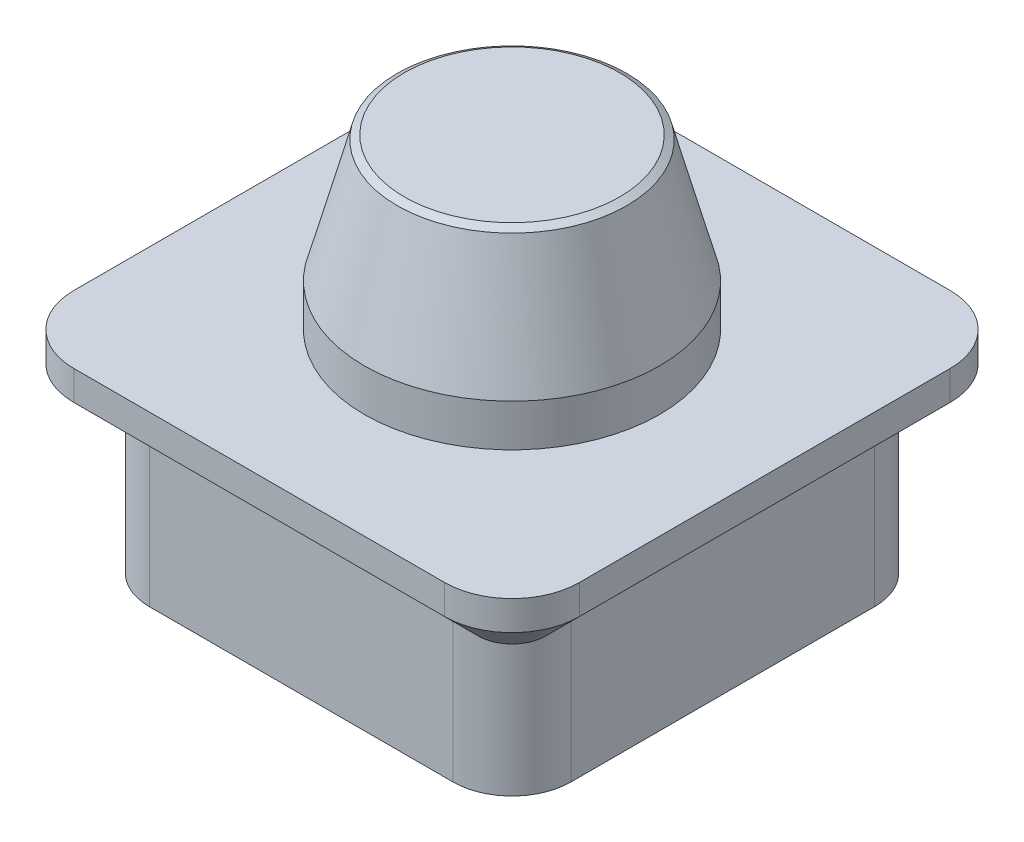
from build123d import *

# Parameters (mm, degrees)
CHAMFER_1_SIZE  = 1
CHAMFER_1_SIZE2 = 1.414213562
EXTRUDE_1_DEPTH = 15
EXTRUDE_2_DEPTH = 35
CHAMFER_2_SIZE  = 8


with BuildPart() as part:
    # 草图1 → 旋转1 (revolve)
    with BuildSketch(Plane.XY, mode=Mode.PRIVATE) as revolve_1_sk:
        Polygon((0, 0), (35, 0), (35, 10), (26.961524227, 40), (0, 40), align=None)
    revolve(revolve_1_sk.sketch.rotate(Axis((0, 40, 0), (0, -1, 0)), 180), axis=Axis((0, 40, 0), (0, -1, 0)))

    # 倒角1
    chamfer_1_edges = [part.edges().sort_by_distance(p)[0] for p in [
        (26.961524227, 40, 0),
    ]]
    chamfer_1_side = [part.faces().sort_by_distance(p)[0] for p in [
        (30.980762114, 25, 0),
    ]]
    chamfer(chamfer_1_edges, length=CHAMFER_1_SIZE, length2=CHAMFER_1_SIZE2, reference=chamfer_1_side[0])

    # 草图2 → 凸台-拉伸1 (add)
    with BuildSketch(Plane.XZ):
        with BuildLine():
            Line((44, -60), (-44, -60))
            ThreePointArc((-44, -60), (-55.313708499, -55.313708499), (-60, -44))
            Line((-60, -44), (-60, 44))
            ThreePointArc((-60, 44), (-55.313708499, 55.313708499), (-44, 60))
            Line((-44, 60), (44, 60))
            ThreePointArc((44, 60), (55.313708499, 55.313708499), (60, 44))
            Line((60, 44), (60, -44))
            ThreePointArc((60, -44), (55.313708499, -55.313708499), (44, -60))
        make_face()
    extrude(amount=EXTRUDE_1_DEPTH)

    # 草图3 → 凸台-拉伸2 (add)
    with BuildSketch(Plane.XZ.offset(15)):
        with BuildLine():
            Line((36, -50), (-36, -50))
            ThreePointArc((-36, -50), (-45.899494937, -45.899494937), (-50, -36))
            Line((-50, -36), (-50, 36))
            ThreePointArc((-50, 36), (-45.899494937, 45.899494937), (-36, 50))
            Line((-36, 50), (36, 50))
            ThreePointArc((36, 50), (45.899494937, 45.899494937), (50, 36))
            Line((50, 36), (50, -36))
            ThreePointArc((50, -36), (45.899494937, -45.899494937), (36, -50))
        make_face()
    extrude(amount=EXTRUDE_2_DEPTH)

    # 倒角2
    chamfer_2_edges = [part.edges().sort_by_distance(p)[0] for p in [
        (-55.313708499, -15, -55.313708499),
        (0, -15, -60),
        (55.313708499, -15, -55.313708499),
        (60, -15, 0),
        (55.313708499, -15, 55.313708499),
        (0, -15, 60),
        (-55.313708499, -15, 55.313708499),
        (-60, -15, 0),
    ]]
    chamfer(chamfer_2_edges, length=CHAMFER_2_SIZE)


solid = part.part
